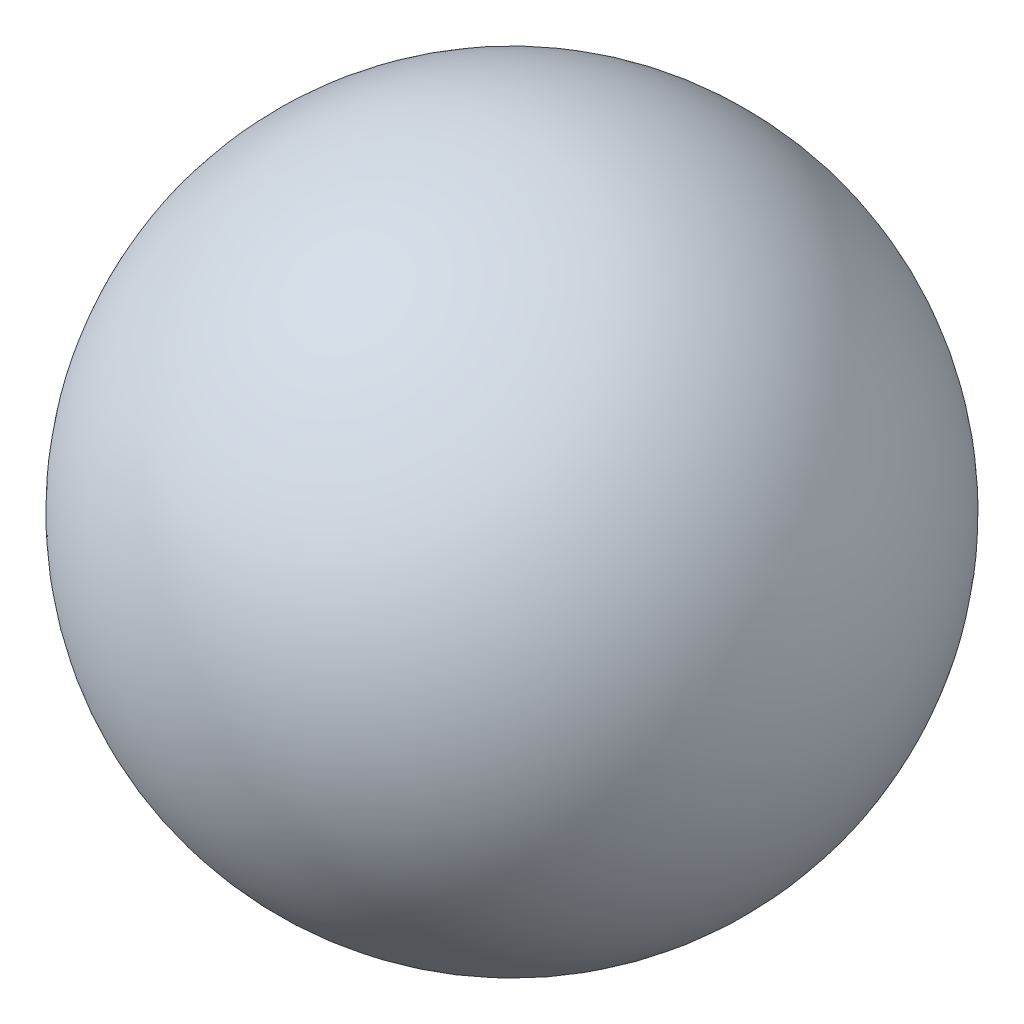
SolidWorks part; units mm, degrees
ref_plane "Front Plane" through (0, 0, 0) normal (0, 0, 1) x (1, 0, 0)
ref_plane "Top Plane" through (0, 0, 0) normal (0, 1, 0) x (1, 0, 0)
ref_plane "Right Plane" through (0, 0, 0) normal (1, 0, 0) x (0, 0, -1)
other "Configuration Table"
sketch "Sketch1" plane through (0, 0, 0) normal (0, 0, 1) x (1, 0, 0)
  line L0 (0, 0) -> (56.0475, 0) construction
  line L1 (29.4, 0) -> (43.1, 0)
  arc A0 (43.1, 0) -> (29.4, 0) centre (36.25, 0) ccw
  dimension "D1" = 13.7
  dimension "D2" = 36.25
revolve "Revolve1" add sketch "Sketch1" angle 360 about L0
